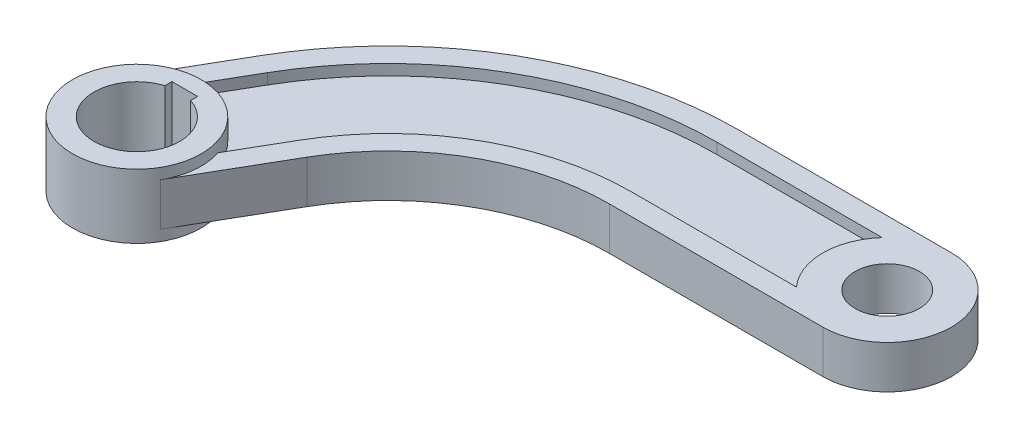
from build123d import *
from build123d.topology import SkipClean

# Parameters (mm, degrees)
SKETCH_1_R          = 30
EXTRUDE_1_DEPTH     = 15
SKETCH_2_R          = 15
EXTRUDE_2_DEPTH     = 10
SKETCH_3_R          = 30
SKETCH_3_R_2        = 15
EXTRUDE_3_DEPTH     = 10
CUT_EXTRUDE_1_DEPTH = 5
CUT_EXTRUDE_START   = -5
CUT_EXTRUDE_2_DEPTH = 5


with BuildPart() as part:
    # 草图1 → 凸台-拉伸1 (new, symmetric)
    with BuildSketch(Plane(origin=(0, 0, 0), x_dir=(1, 0, 0), z_dir=(0, 1, 0))):
        with Locations(Location((0, 0, 0), (0, 0, 270))):
            Circle(SKETCH_1_R)
        with BuildLine():
            Line((6, 19.078784028), (6, 22.378784028))
            Line((6, 22.378784028), (-6, 22.378784028))
            Line((-6, 22.378784028), (-6, 19.078784028))
            ThreePointArc((-6, 19.078784028), (0, -20), (6, 19.078784028))
        make_face(mode=Mode.SUBTRACT)
    extrude(amount=EXTRUDE_1_DEPTH, both=True)

    # 草图2 → 凸台-拉伸2 (add, symmetric)
    with BuildSketch(Plane(origin=(0, 0, 0), x_dir=(1, 0, 0), z_dir=(0, 1, 0))):
        with BuildLine():
            Line((-25.980762114, 15), (-0.980762114, 58.301270189))
            ThreePointArc((-0.980762114, 58.301270189), (58.826859022, 118.108891325), (140.525588833, 140))
            Line((140.525588833, 140), (240, 140))
            ThreePointArc((240, 140), (270, 110), (240, 80))
            Line((240, 80), (140.525588833, 80))
            ThreePointArc((140.525588833, 80), (88.826859022, 66.147367097), (50.980762114, 28.301270189))
            Line((50.980762114, 28.301270189), (25.980762114, -15))
            ThreePointArc((25.980762114, -15), (15, 25.980762114), (-25.980762114, 15))
        make_face()
        with Locations(Location((240, 110, 0), (0, 0, 270))):
            Circle(SKETCH_2_R, mode=Mode.SUBTRACT)
    extrude(amount=EXTRUDE_2_DEPTH, both=True)

    # 草图3 → 凸台-拉伸3 (add, symmetric)
    with BuildSketch(Plane(origin=(0, 0, 0), x_dir=(1, 0, 0), z_dir=(0, 1, 0))):
        with Locations((240, 110)):
            Circle(SKETCH_3_R)
        with Locations(Location((240, 110, 0), (0, 0, 270))):
            Circle(SKETCH_3_R_2, mode=Mode.SUBTRACT)
    extrude(amount=EXTRUDE_3_DEPTH, both=True)

    # 草图4 → 切除-拉伸1 (cut)
    with SkipClean():  # the faces are left unmerged after this step: merging them gives an invalid solid
        with BuildSketch(Plane(origin=(0, 10, 0), x_dir=(1, 0, 0), z_dir=(0, 1, 0))):
            with BuildLine():
                Line((217.639320225, 130), (140.525588833, 130))
                ThreePointArc((140.525588833, 130), (63.826859022, 109.448637287), (7.679491924, 53.301270189))
                Line((7.679491924, 53.301270189), (-6.140168188, 29.364916731))
                ThreePointArc((-6.140168188, 29.364916731), (15, 25.980762114), (28.500847963, 9.364916731))
                Line((28.500847963, 9.364916731), (42.320508076, 33.301270189))
                ThreePointArc((42.320508076, 33.301270189), (83.826859022, 74.807621135), (140.525588833, 90))
                Line((140.525588833, 90), (217.639320225, 90))
                ThreePointArc((217.639320225, 90), (210, 110), (217.639320225, 130))
            make_face()
        extrude(amount=-CUT_EXTRUDE_1_DEPTH, mode=Mode.SUBTRACT)

    # 草图5 → 切除-拉伸2 (cut)
    with SkipClean():  # the faces are left unmerged after this step: merging them gives an invalid solid
        with BuildSketch(Plane.XZ.offset(10).offset(CUT_EXTRUDE_START)):
            with BuildLine():
                Line((217.639320225, -90), (140.525588833, -90))
                ThreePointArc((140.525588833, -90), (83.826859022, -74.807621135), (42.320508076, -33.301270189))
                Line((42.320508076, -33.301270189), (28.500847963, -9.364916731))
                ThreePointArc((28.500847963, -9.364916731), (15, -25.980762114), (-6.140168188, -29.364916731))
                Line((-6.140168188, -29.364916731), (7.679491924, -53.301270189))
                ThreePointArc((7.679491924, -53.301270189), (63.826859022, -109.448637287), (140.525588833, -130))
                Line((140.525588833, -130), (217.639320225, -130))
                ThreePointArc((217.639320225, -130), (210, -110), (217.639320225, -90))
            make_face()
        extrude(amount=CUT_EXTRUDE_2_DEPTH, mode=Mode.SUBTRACT)


solid = part.part
